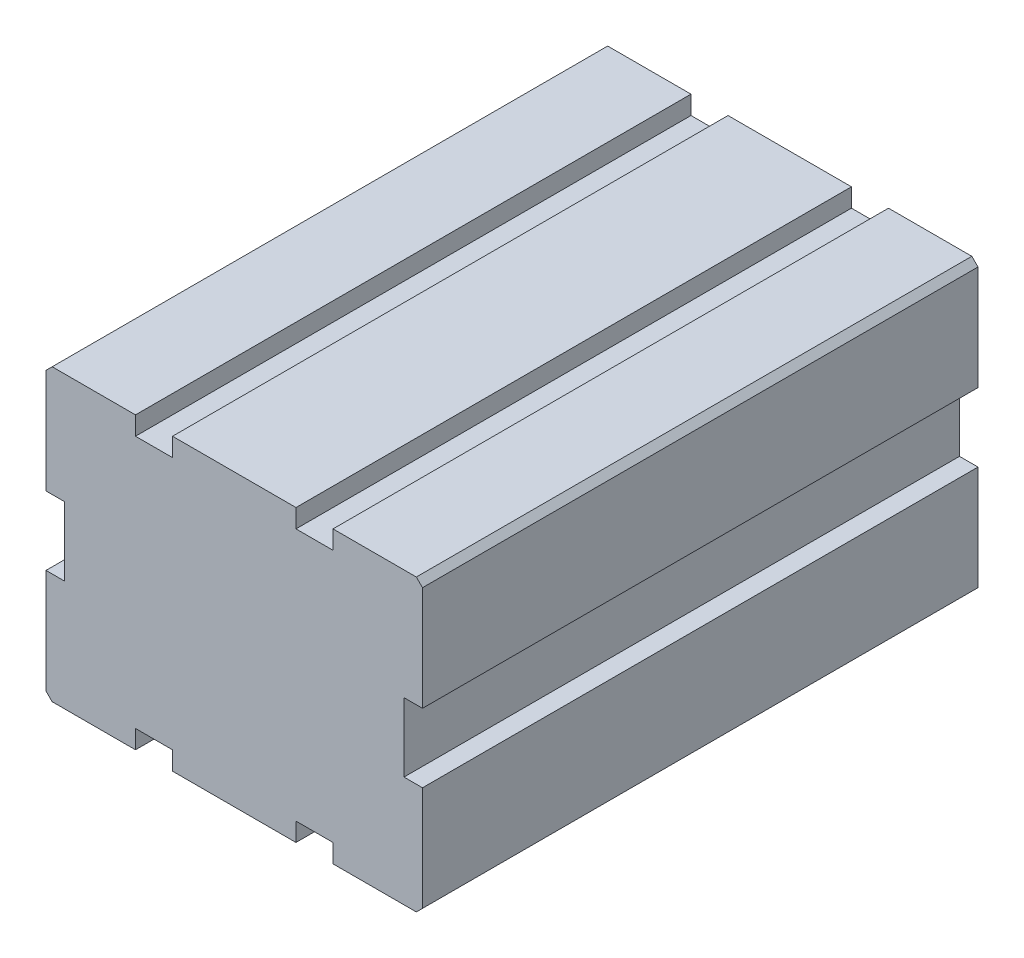
SolidWorks part; units mm, degrees
ref_plane "Front Plane" through (0, 0, 0) normal (0, 0, 1) x (1, 0, 0)
ref_plane "Top Plane" through (0, 0, 0) normal (0, 1, 0) x (1, 0, 0)
ref_plane "Right Plane" through (0, 0, 0) normal (1, 0, 0) x (0, 0, -1)
sketch "Sketch1" plane through (0, 0, 0) normal (0, 0, 1) x (1, 0, 0)
  line L0 (-15.25, 11.25) -> (-14.75, 11.75)
  line L1 (-14.75, 11.75) -> (-8, 11.75)
  line L2 (-15.25, 11.25) -> (-15.25, 2.7865)
  line L3 (-14.75, -11.75) -> (-8, -11.75)
  line L4 (15.25, 11.25) -> (15.25, 2.7865)
  line L5 (-15.25, 11.75) -> (15.25, -11.75) construction
  line L6 (-15.25, -11.75) -> (15.25, 11.75) construction
  line L11 (14.75, 11.75) -> (15.25, 11.25)
  line L12 (14.75, -11.75) -> (15.25, -11.25)
  line L13 (-15.25, -11.25) -> (-14.75, -11.75)
  line L14 (0, 39.9588) -> (0, -61.159) construction
  line L15 (-31.9889, 0) -> (30.5933, 0) construction
  line L16 (-8, 11.75) -> (-8, 10.25)
  line L17 (-8, 10.25) -> (-5, 10.25)
  line L18 (-5, 10.25) -> (-5, 11.75)
  line L19 (5, 10.25) -> (5, 11.75)
  line L20 (8, 11.75) -> (8, 10.25)
  line L21 (8, 10.25) -> (5, 10.25)
  line L22 (8, -11.75) -> (8, -10.25)
  line L23 (8, -10.25) -> (5, -10.25)
  line L24 (5, -10.25) -> (5, -11.75)
  line L25 (-5, -10.25) -> (-5, -11.75)
  line L26 (-8, -10.25) -> (-5, -10.25)
  line L27 (-8, -11.75) -> (-8, -10.25)
  line L28 (-5, 11.75) -> (5, 11.75)
  line L29 (8, 11.75) -> (14.75, 11.75)
  line L30 (8, -11.75) -> (14.75, -11.75)
  line L31 (-5, -11.75) -> (5, -11.75)
  line L32 (15.25, 2.7865) -> (13.75, 2.7865)
  line L33 (13.75, 2.7865) -> (13.75, -2.7865)
  line L34 (15.25, -2.7865) -> (13.75, -2.7865)
  line L35 (15.25, -2.7865) -> (15.25, -11.25)
  line L36 (-15.25, -2.7865) -> (-13.75, -2.7865)
  line L37 (-15.25, 2.7865) -> (-13.75, 2.7865)
  line L38 (-13.75, 2.7865) -> (-13.75, -2.7865)
  line L39 (-15.25, -2.7865) -> (-15.25, -11.25)
  point P0 (0, 0)
  point P38 (13.75, 0)
  dimension "D1" = 30.5
  dimension "D2" = 23.5
  dimension "D3" = 5
  dimension "D4" = 3
  dimension "D9" = 1.5
  dimension "D10" = 1.5
extrude "Boss-Extrude2" add sketch "Sketch1" along normal blind 45
